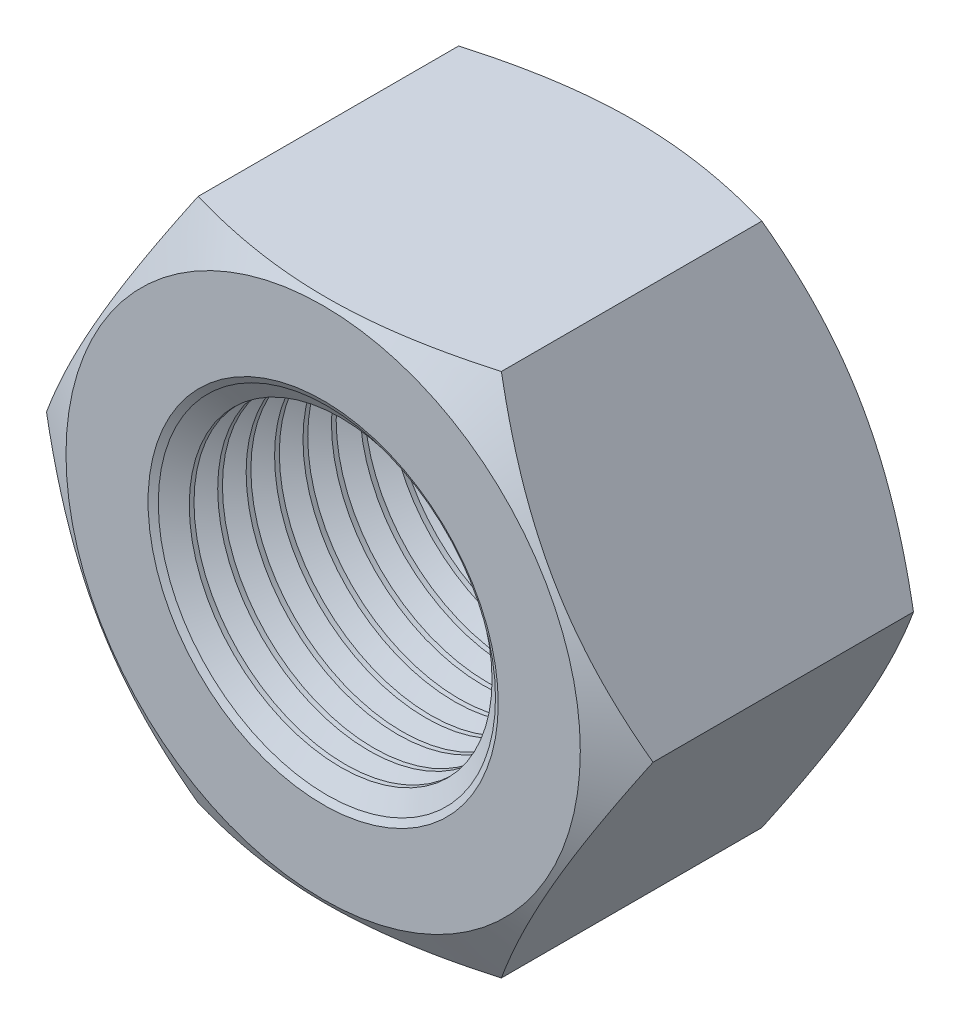
from build123d import *
from OCP.BRepFilletAPI import BRepFilletAPI_MakeChamfer

# Parameters (mm, degrees)
SKETCH1_R        = 10.376
BASENUT_DEPTH    = 21.5
ENDCHAMFER_SIZE  = 1.624
ENDCHAMFER_SIZE2 = 0.937616837
LPATTERN10_COUNT = 11
LPATTERN10_PITCH = 1.9488


with BuildPart() as part:
    # Sketch1 → BaseNut (new body)
    with BuildSketch(Plane.XY):
        Polygon((20.784609691, 0), (10.392304845, 18), (-10.392304845, 18), (-20.784609691, 0), (-10.392304845, -18), (10.392304845, -18), align=None)
        Circle(SKETCH1_R, mode=Mode.SUBTRACT)
    extrude(amount=-BASENUT_DEPTH)

    # Sketch2 → Double-Chamfer (revolve, cut)
    with BuildSketch(Plane(origin=(0, 0, 0), x_dir=(1, 0, 0), z_dir=(0, 1, 0))):
        Polygon((-20.784609691, 21.5), (-17.625, 21.5), (-20.784609691, 19.675798494), align=None)
        Polygon((-20.784609691, 1.824201506), (-20.784609691, 0), (-17.625, 0), align=None)
    revolve(axis=Axis((0, 0, -3.375940562), (0, 0, 1)), mode=Mode.SUBTRACT)

    # EndChamfer: one chamfer whose edges measure the first distance from different faces: ONE call of the kernel's chamfer builder (chamfer() names one face for all edges)
    endchamfer_edges_1 = [part.edges().sort_by_distance(p)[0] for p in [
        (-10.376, 0, -21.5),
    ]]
    endchamfer_side_1 = [part.faces().sort_by_distance(p)[0] for p in [
        (-10.376, 0, -10.75),
    ]]
    endchamfer_edges_2 = [part.edges().sort_by_distance(p)[0] for p in [
        (-10.376, 0, 0),
    ]]
    endchamfer_side_2 = [part.faces().sort_by_distance(p)[0] for p in [
        (17.126489719, 0, 0),
    ]]
    endchamfer = BRepFilletAPI_MakeChamfer(part.part.solid().wrapped)
    for e in endchamfer_edges_1:
        endchamfer.Add(ENDCHAMFER_SIZE, ENDCHAMFER_SIZE2, e.wrapped, endchamfer_side_1[0].wrapped)  # the first distance lies on this face
    for e in endchamfer_edges_2:
        endchamfer.Add(ENDCHAMFER_SIZE, ENDCHAMFER_SIZE2, e.wrapped, endchamfer_side_2[0].wrapped)  # the first distance lies on this face
    add(Compound.cast(endchamfer.Shape()), mode=Mode.REPLACE)

    # Sketch3 → Cut-Revolve10 (revolve, cut)
    with BuildSketch(Plane(origin=(0, 0, 0), x_dir=(1, 0, 0), z_dir=(0, 1, 0)), mode=Mode.PRIVATE) as cut_revolve10_sk:
        Polygon((-11.782425256, 19.876), (-10.376, 19.064), (-8.752, 19.064), (-8.752, 20.688), (-10.376, 20.688), align=None)
    cut_revolve10 = revolve(cut_revolve10_sk.sketch.rotate(Axis((0, 0, -7.438254559), (0, 0, -1)), 180), axis=Axis((0, 0, -7.438254559), (0, 0, -1)), mode=Mode.SUBTRACT)

    # LPattern10: Cut-Revolve10 ×11
    with Locations(*[(0, 0, i * LPATTERN10_PITCH) for i in range(1, LPATTERN10_COUNT)]):
        add(cut_revolve10, mode=Mode.SUBTRACT)


solid = part.part
